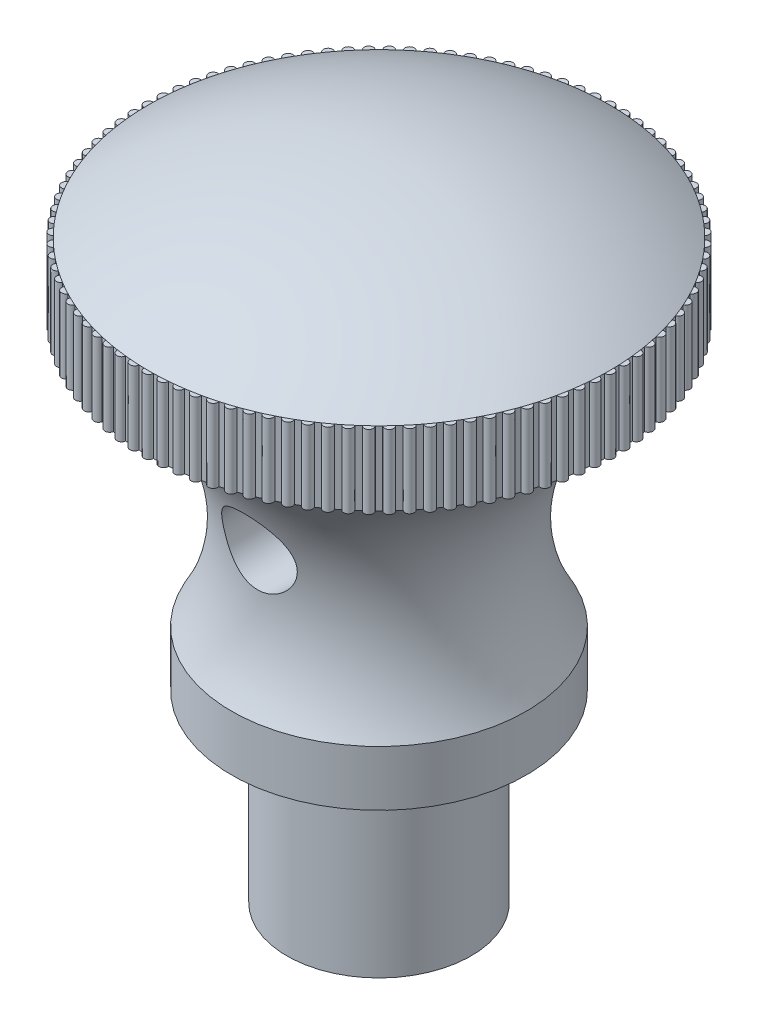
SolidWorks part; units mm, degrees
ref_plane "Front Plane" through (0, 0, 0) normal (0, 0, 1) x (1, 0, 0)
ref_plane "Top Plane" through (0, 0, 0) normal (0, 1, 0) x (1, 0, 0)
ref_plane "Right Plane" through (0, 0, 0) normal (1, 0, 0) x (0, 0, -1)
sketch "Sketch7" plane through (0, 0, 0) normal (0, 0, 1) x (1, 0, 0)
  line L0 (0, 0) -> (0, 42.1867) construction
  line L1 (0, 35) -> (0, 0)
  line L2 (0, 0) -> (5, 0)
  line L3 (5, 0) -> (5, 10)
  line L4 (5, 10) -> (8, 10)
  line L5 (8, 10) -> (8, 13)
  line L6 (12.5, 31.255) -> (12.5, 27.255)
  arc A0 (8, 13) -> (12.5, 27.255) centre (16.5853, 18.1276) cw
  arc A1 (0, 35) -> (12.5, 31.255) centre (0, 12.2663) cw
  dimension "D6" = 10
  dimension "D1" = 35
  dimension "D2" = 5
  dimension "D3" = 3
  dimension "D4" = 3
  dimension "D5" = 10
  dimension "D7" = 4
  dimension "D8" = 12.5
revolve "Revolve3" add sketch "Sketch7" angle 360 about L0
cosmetic thread "Cosmetic Thread3" parameters "D2"=9
sketch "Sketch8" plane through (0, 0, 0) normal (0, 0, 1) x (1, 0, 0)
  line L0 (-5, 0) -> (5, 0) construction
  circle A0 centre (0, 20) radius 2
  dimension "D1" = 20
extrude "Cut-Extrude4" cut sketch "Sketch8" against normal mid plane 20
ref_plane "Plane5" through (0, 27.255, 0) normal (0, -1, 0) x (-1, 0, 0)
sketch "Sketch9" plane through (0, 27.255, 0) normal (0, -1, 0) x (-1, 0, 0)
  circle A0 centre (-12.5, 0) radius 0.25
  circle A1 centre (0, 0) radius 12.5 construction
extrude "Boss-Extrude2" add sketch "Sketch9" against normal blind 4
pattern_circular "CirPattern3" count 100 over 360 about axis through (0, 0, 0) along (0, 1, 0) of "Boss-Extrude2"
sketch "Sketch10" plane through (0, 0, 0) normal (0, -1, 0) x (1, 0, 0)
  circle A0 centre (0, 0) radius 2
extrude "Cut-Extrude6" cut sketch "Sketch10" against normal blind 22
